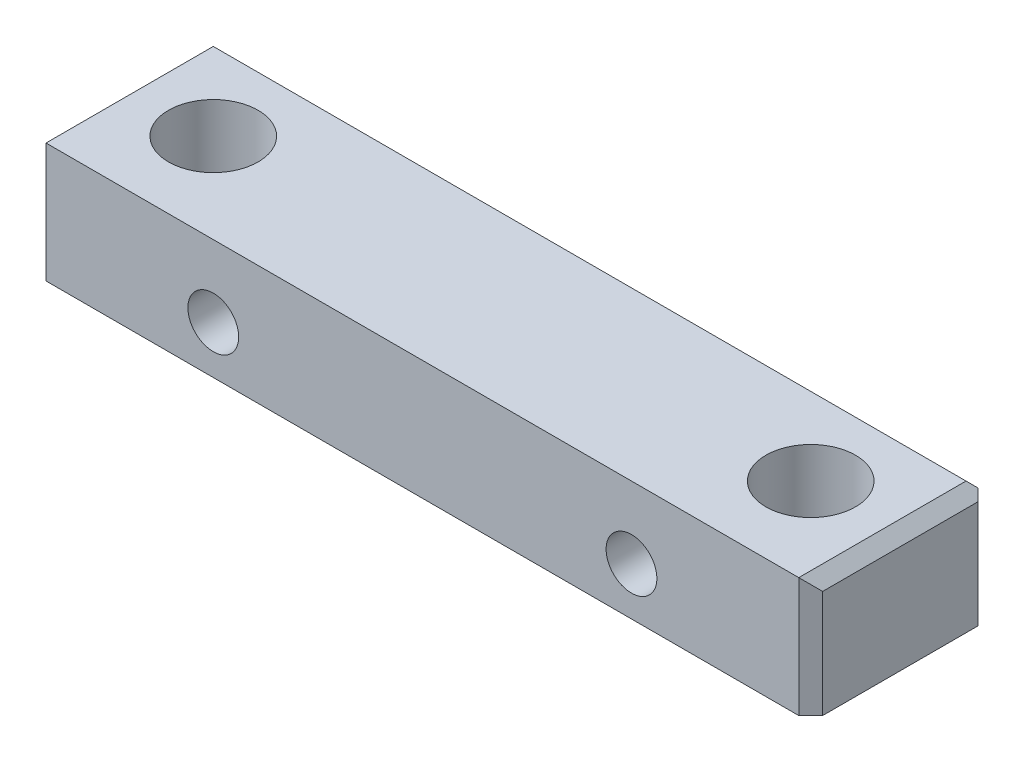
from build123d import *

# Parameters (mm, degrees)
SKETCH_1_W                = 130
SKETCH_1_H                = 20
EXTRUDE_1_DEPTH           = 30
HOLE_WIZARD_1_D           = 9
HOLE_WIZARD_1_CBORE_D     = 15
HOLE_WIZARD_1_CBORE_DEPTH = 15
HOLE_WIZARD_M10_1_D       = 8.5
CHAMFER_1_SIZE            = 2
CHAMFER_2_SIZE            = 2


with BuildPart() as part:
    # 草图1 → 凸台-拉伸1 (new body)
    with BuildSketch(Plane.XY):
        Rectangle(SKETCH_1_W, SKETCH_1_H)
    extrude(amount=EXTRUDE_1_DEPTH)

    # 打孔尺寸(%根据)内六角圆柱头螺钉的类型1 (through all)
    with Locations(Plane(origin=(0, 10, 0), x_dir=(1, 0, 0), z_dir=(0, 1, 0))):
        with Locations((-50, -15), (50, -15)):
            CounterBoreHole(HOLE_WIZARD_1_D / 2, HOLE_WIZARD_1_CBORE_D / 2, HOLE_WIZARD_1_CBORE_DEPTH)

    # M10 螺纹孔1 (through all)
    with Locations(Plane.XY.offset(30)):
        with Locations((-35, -2), (35, -2)):
            Hole(HOLE_WIZARD_M10_1_D / 2)

    # 倒角1
    chamfer_1_edges = [part.edges().sort_by_distance(p)[0] for p in [
        (-65, 0, 30),
        (65, 0, 30),
        (-65, 0, 0),
        (65, 0, 0),
        (-65, 10, 15),
        (65, 10, 15),
    ]]
    chamfer(chamfer_1_edges, length=CHAMFER_1_SIZE)

    # 倒角2
    chamfer_2_edges = [part.edges().sort_by_distance(p)[0] for p in [
        (0, 10, 0),
    ]]
    chamfer(chamfer_2_edges, length=CHAMFER_2_SIZE)


solid = part.part
